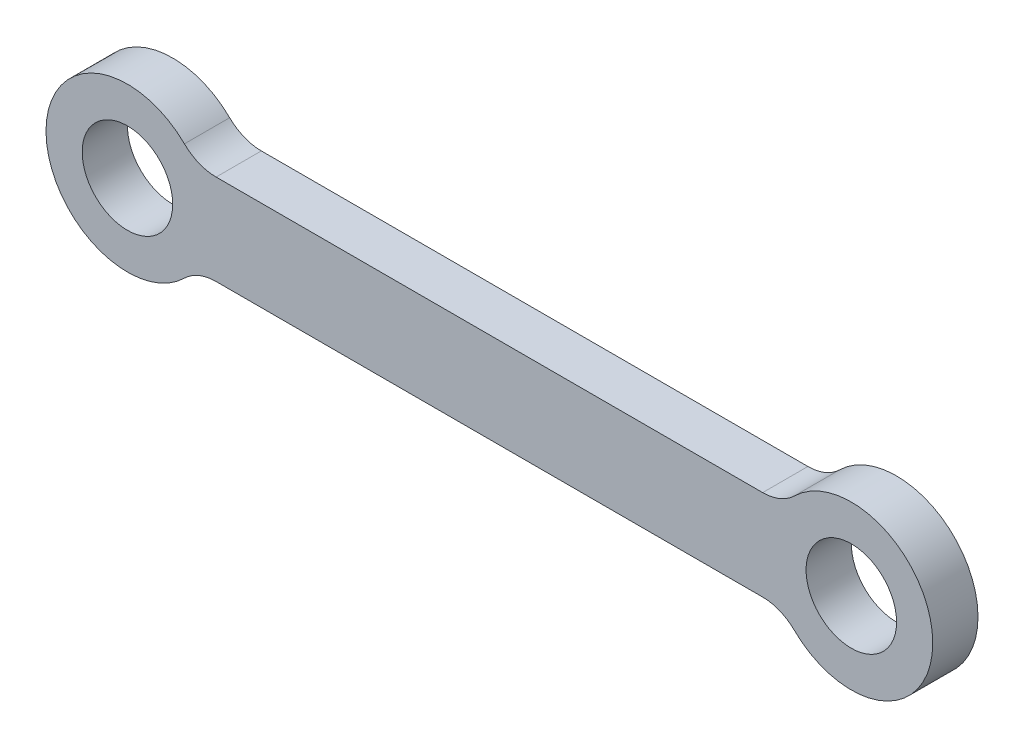
SolidWorks part; units mm, degrees
ref_plane "Front Plane" through (0, 0, 0) normal (0, 0, 1) x (1, 0, 0)
ref_plane "Top Plane" through (0, 0, 0) normal (0, 1, 0) x (1, 0, 0)
ref_plane "Right Plane" through (0, 0, 0) normal (1, 0, 0) x (0, 0, -1)
sketch "Sketch1" plane through (0, 0, 0) normal (0, 0, 1) x (1, 0, 0)
  line L0 (9.798, 5) -> (70.202, 5)
  line L1 (9.798, -5) -> (70.202, -5)
  circle A0 centre (0, 0) radius 5
  arc A1 (6.2987, 6.4286) -> (6.2987, -6.4286) centre (0, 0) ccw
  circle A2 centre (80, 0) radius 5
  arc A3 (73.7013, -6.4286) -> (73.7013, 6.4286) centre (80, 0) ccw
  arc A4 (70.202, 5) -> (73.7013, 6.4286) centre (70.202, 10) ccw
  arc A5 (70.202, -5) -> (73.7013, -6.4286) centre (70.202, -10) cw
  arc A6 (9.798, -5) -> (6.2987, -6.4286) centre (9.798, -10) ccw
  arc A7 (9.798, 5) -> (6.2987, 6.4286) centre (9.798, 10) cw
  dimension "D1" = 10
  dimension "D3" = 18
  dimension "D4" = 5
  dimension "D2" = 80
extrude "Boss-Extrude1" add sketch "Sketch1" along normal blind 5
